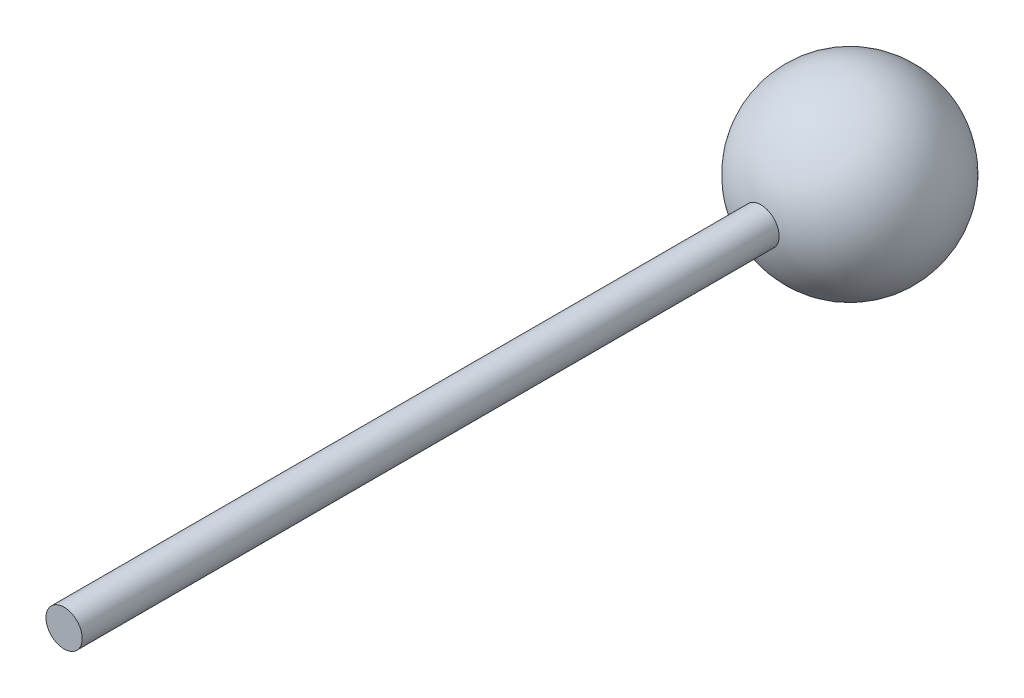
SolidWorks part; units mm, degrees
ref_plane "Front Plane" through (0, 0, 0) normal (0, 0, 1) x (1, 0, 0)
ref_plane "Top Plane" through (0, 0, 0) normal (0, 1, 0) x (1, 0, 0)
ref_plane "Right Plane" through (0, 0, 0) normal (1, 0, 0) x (0, 0, -1)
sketch "Sketch1" plane through (0, 0, 0) normal (0, 1, 0) x (1, 0, 0)
  line L0 (0, -1000) -> (0, 49000) construction
  line L1 (0, 15) -> (0, -15)
  arc A0 (0, 15) -> (0, -15) centre (0, 0) ccw
  dimension "D1" = 30
revolve "Revolve3" add sketch "Sketch1" angle 360 about L0
sketch "Sketch2" plane through (0, 0, 0) normal (0, 0, 1) x (1, 0, 0)
  circle A0 centre (0, 0) radius 3
  dimension "D1" = 6
extrude "Boss-Extrude1" add sketch "Sketch2" along normal blind 130
